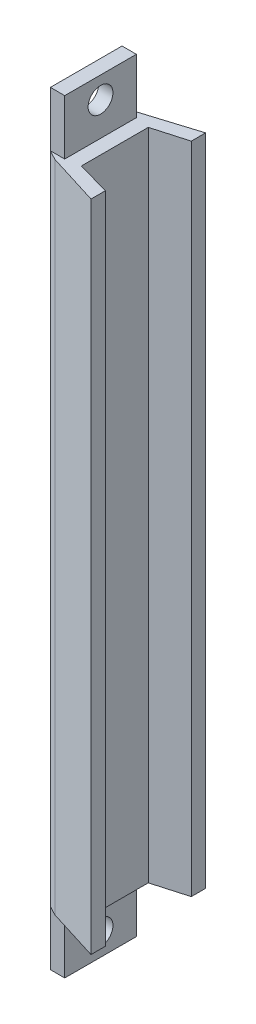
from build123d import *

# Parameters (mm, degrees)
BOSS_EXTRUDE1_DEPTH = 342.5
SKETCH2_W           = 15
SKETCH2_H           = 75
BOSS_EXTRUDE2_DEPTH = 57.5
SKETCH3_R           = 13
CUT_EXTRUDE1_DEPTH  = 57.5


with BuildPart() as part:
    # Sketch1 → Boss-Extrude1 (new, symmetric)
    with BuildSketch(Plane(origin=(0, 0, 0), x_dir=(1, 0, 0), z_dir=(0, 1, 0))):
        Polygon((0, -37.5), (0, 37.5), (10, 42.881796684), (65, 60), (65, 45), (30, 35), (30, -35), (65, -45), (65, -60), (10, -42.881796684), align=None)
    extrude(amount=BOSS_EXTRUDE1_DEPTH, both=True)

    # Sketch2 → Boss-Extrude2 (add)
    with BuildSketch(Plane.XZ.offset(342.5)):
        with Locations((7.5, 0)):
            Rectangle(SKETCH2_W, SKETCH2_H)
    boss_extrude2 = extrude(amount=BOSS_EXTRUDE2_DEPTH)

    # Mirror1: Boss-Extrude2 across plane
    add(boss_extrude2.mirror(Plane.ZX))

    # Sketch3 → Cut-Extrude1 (cut)
    with BuildSketch(Plane.ZY):
        with Locations((0, 377.5)):
            Circle(SKETCH3_R)
        with Locations((0, -377.5)):
            Circle(SKETCH3_R)
    extrude(amount=-CUT_EXTRUDE1_DEPTH, mode=Mode.SUBTRACT)


solid = part.part
